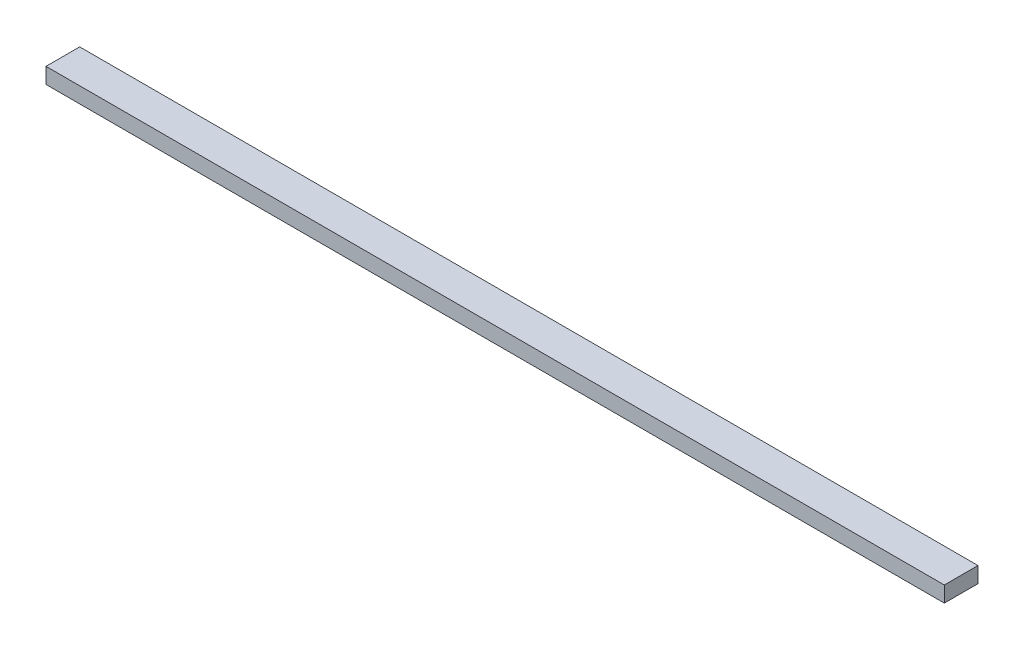
SolidWorks part; units mm, degrees
ref_plane "前视基准面" through (0, 0, 0) normal (0, 0, 1) x (1, 0, 0)
ref_plane "上视基准面" through (0, 0, 0) normal (0, 1, 0) x (1, 0, 0)
ref_plane "右视基准面" through (0, 0, 0) normal (1, 0, 0) x (0, 0, -1)
sketch "草图1" plane through (0, 0, 0) normal (0, 0, 1) x (1, 0, 0)
  line L1 (-400, -7) -> (400, -7)
  line L2 (-400, -7) -> (-400, 7)
  line L3 (-400, 7) -> (400, 7)
  line L4 (400, -7) -> (400, 7)
  line L5 (-400, -7) -> (400, 7) construction
  line L6 (-400, 7) -> (400, -7) construction
  point P0 (0, 0)
  dimension "D1" = 14
  dimension "D2" = 800
extrude "凸台-拉伸1" add sketch "草图1" along normal blind 30
